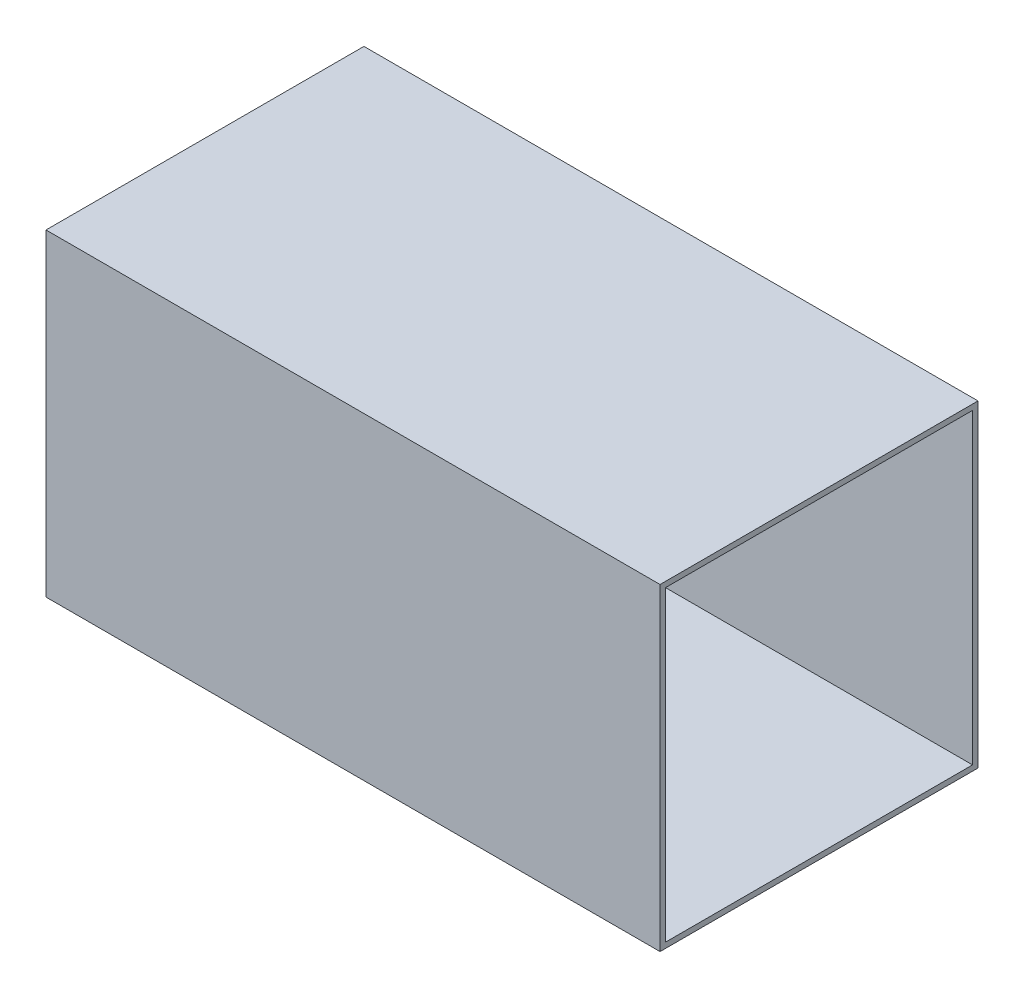
from build123d import *

# Parameters (mm, degrees)
SKETCH1_W           = 466
SKETCH1_H           = 466
SKETCH1_W_2         = 450
SKETCH1_H_2         = 450
BOSS_EXTRUDE1_DEPTH = 900


with BuildPart() as part:
    # Sketch1 → Boss-Extrude1 (new body)
    with BuildSketch(Plane(origin=(0, 0, 0), x_dir=(0, 0, -1), z_dir=(1, 0, 0))):
        Rectangle(SKETCH1_W, SKETCH1_H)
        Rectangle(SKETCH1_W_2, SKETCH1_H_2, mode=Mode.SUBTRACT)
    extrude(amount=BOSS_EXTRUDE1_DEPTH)


solid = part.part
